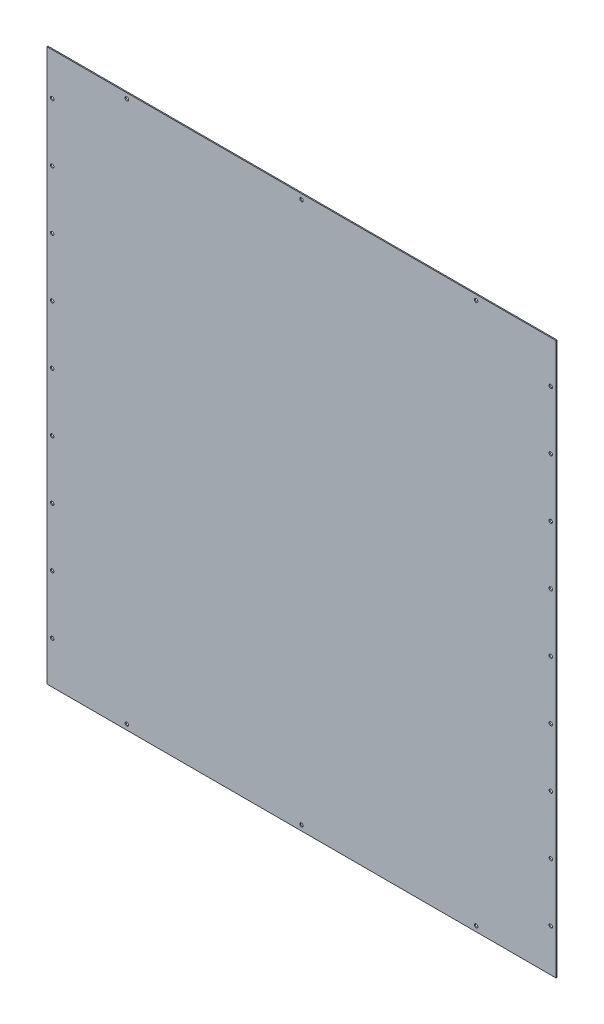
SolidWorks part; units mm, degrees
material "304"
ref_plane "前视基准面" through (0, 0, 0) normal (0, 0, 1) x (1, 0, 0)
ref_plane "上视基准面" through (0, 0, 0) normal (0, 1, 0) x (1, 0, 0)
ref_plane "右视基准面" through (0, 0, 0) normal (1, 0, 0) x (0, 0, -1)
sketch "草图1" plane through (0, 0, 0) normal (0, 0, 1) x (1, 0, 0)
  line L0 (0, 0) -> (451.2544, 0) construction
  line L1 (-481, 521.5) -> (481, 521.5)
  line L2 (-481, 521.5) -> (-481, -521.5)
  line L3 (-481, -521.5) -> (481, -521.5)
  line L4 (481, 521.5) -> (481, -521.5)
  line L5 (-481, 521.5) -> (481, -521.5) construction
  line L6 (-481, -521.5) -> (481, 521.5) construction
  line L7 (0, 0) -> (0, 412.8629) construction
  circle A0 centre (-471, 0) radius 3.25
  circle A1 centre (-471, -110.375) radius 3.25
  circle A2 centre (-471, -220.75) radius 3.25
  circle A3 centre (-471, -331.125) radius 3.25
  circle A4 centre (-471, -441.5) radius 3.25
  circle A34 centre (0, -511.5) radius 3.25
  circle A35 centre (0, 511.5) radius 3.25
  circle A36 centre (-471, 441.5) radius 3.25
  circle A37 centre (-471, 331.125) radius 3.25
  circle A38 centre (-471, 220.75) radius 3.25
  circle A39 centre (-471, 110.375) radius 3.25
  circle A40 centre (471, 110.375) radius 3.25
  circle A41 centre (471, 220.75) radius 3.25
  circle A42 centre (471, 331.125) radius 3.25
  circle A43 centre (471, 441.5) radius 3.25
  circle A44 centre (471, -441.5) radius 3.25
  circle A45 centre (471, -331.125) radius 3.25
  circle A46 centre (471, -220.75) radius 3.25
  circle A47 centre (471, -110.375) radius 3.25
  circle A48 centre (471, 0) radius 3.25
  circle A49 centre (330, -511.5) radius 3.25
  circle A50 centre (-330, -511.5) radius 3.25
  circle A51 centre (-330, 511.5) radius 3.25
  circle A52 centre (330, 511.5) radius 3.25
  point P0 (0, 0)
  dimension "D3" = 6.5
  dimension "D8" = 660
  dimension "D1" = 962
  dimension "D2" = 1043
  dimension "D4" = 10
  dimension "D6" = 10
  dimension "D7" = 80
  dimension "D5" = 5
extrude "凸台-拉伸1" add sketch "草图1" along normal blind 2
sketch "草图2" plane through (0, -521.5, 0) normal (0, -1, 0) x (1, 0, 0)
  line L0 (-481, 2) -> (481, 2) construction
  line L1 (481, 0) -> (478.5, 0)
  line L2 (481, 0) -> (481, 2)
  line L3 (481, 2) -> (478.5, 2)
  line L4 (478.5, 0) -> (478.5, 2)
  line L5 (481, 0) -> (478.5, 2) construction
  line L6 (481, 2) -> (478.5, 0) construction
  point P4 (479.75, 1)
  dimension "D1" = 2.5
